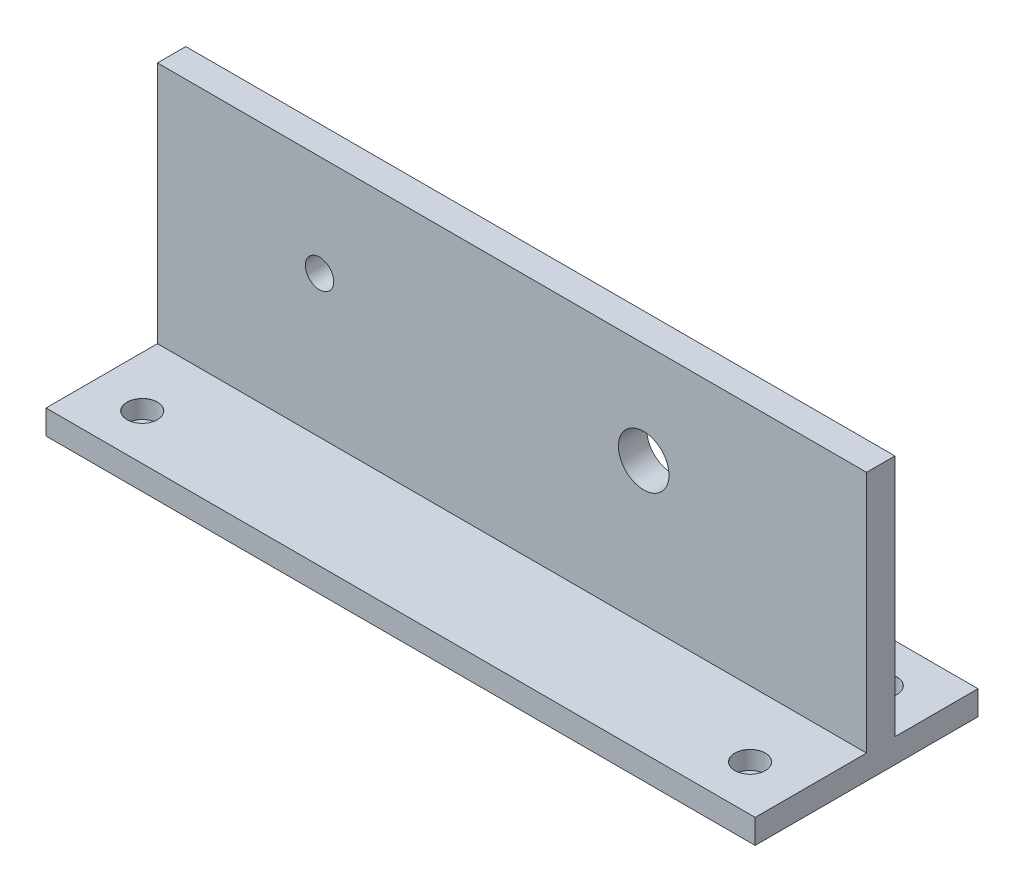
SolidWorks part; units mm, degrees
ref_plane "Front Plane" through (0, 0, 0) normal (0, 0, 1) x (1, 0, 0)
ref_plane "Top Plane" through (0, 0, 0) normal (0, 1, 0) x (1, 0, 0)
ref_plane "Right Plane" through (0, 0, 0) normal (1, 0, 0) x (0, 0, -1)
other "Configuration Table"
sketch "Sketch1" plane through (0, 0, 0) normal (0, 1, 0) x (1, 0, 0)
  line L1 (-175, -55) -> (175, -55)
  line L2 (-175, -55) -> (-175, 55)
  line L3 (-175, 55) -> (175, 55)
  line L4 (175, -55) -> (175, 55)
  line L5 (-175, -55) -> (175, 55) construction
  line L6 (-175, 55) -> (175, -55) construction
  point P0 (0, 0)
  dimension "D1" = 110
  dimension "D2" = 350
extrude "Boss-Extrude1" add sketch "Sketch1" along normal blind 12
sketch "Sketch2" plane through (0, 12, 0) normal (0, 1, 0) x (1, 0, 0)
  line L0 (-175, 55) -> (-175, -55) construction
  line L1 (-175, 14) -> (175, 14)
  line L2 (-175, 14) -> (-175, 0)
  line L3 (-175, 0) -> (175, 0)
  line L4 (175, 14) -> (175, 0)
  line L5 (175, -55) -> (175, 55) construction
  dimension "D1" = 14
extrude "Boss-Extrude2" add sketch "Sketch2" along normal blind 120
hole_wizard "CBORE for M8 Hexagon socket head cap screws1" positions "Sketch5" profile "Sketch4" counterbore size "M8" standard "GB"
sketch "Sketch5" plane through (0, 12, 0) normal (0, 1, 0) x (1, 0, 0)
  line L0 (-150, 32.5) -> (-150, -32.5) construction
  line L2 (150, 32.5) -> (150, -32.5) construction
  point P0 (-150, 32.5)
  point P2 (-150, -32.5)
  point P4 (150, 32.5)
  point P6 (150, -32.5)
  dimension "D1" = 65
  dimension "D2" = 32.5
  dimension "D3" = 32.5
  dimension "D4" = 65
  dimension "D5" = 300
  dimension "D6" = 150
sketch "Sketch4" plane through (-150, 12, -32.5) normal (1, 0, 0) x (0, 0, 1)
  line L0 (0, 0) -> (0, 15.1039)
  line L1 (0, 15.1039) -> (4.5, 12.4)
  line L2 (4.5, 12.4) -> (4.5, 9)
  line L3 (4.5, 9) -> (7.5, 9)
  line L5 (7.5, 9) -> (7.5, 0.025)
  line L6 (7.5, 0.025) -> (7.525, 0)
  line L7 (7.525, 0) -> (0, 0)
  line L8 (-7.5, 0.025) -> (-7.525, 0) construction
  line L10 (0, 15.1039) -> (-4.5, 12.4) construction
  line L11 (0, -6.35) -> (0, 107.95) construction
  dimension "孔直径" = 9
  dimension "孔深度" = 12.4
  dimension "锥形沉头孔直径" = 15
  dimension "锥形沉头孔深度" = 9
  dimension "近端锥形沉头孔直径" = 15.05
  dimension "近端锥形沉头孔角度" = 90
  dimension "导头角度" = 118
sketch "Sketch6" plane through (0, 0, -14) normal (0, 0, -1) x (-1, 0, 0)
  line L0 (-175, 132) -> (175, 132) construction
  line L1 (175, 132) -> (175, 12) construction
  circle A0 centre (95, 82) radius 7
  dimension "D1" = 14
  dimension "D2" = 50
  dimension "D3" = 80
extrude "Cut-Extrude1" cut sketch "Sketch6" against normal through all both and the other way through all
sketch "Sketch7" plane through (0, 0, -14) normal (0, 0, -1) x (-1, 0, 0)
  line L0 (-175, 132) -> (175, 132) construction
  line L1 (-175, 132) -> (-175, 12) construction
  circle A0 centre (-65, 82) radius 12.5
  dimension "D1" = 50
  dimension "D2" = 25
  dimension "D3" = 110
extrude "Cut-Extrude2" cut sketch "Sketch7" against normal through all both and the other way through all
